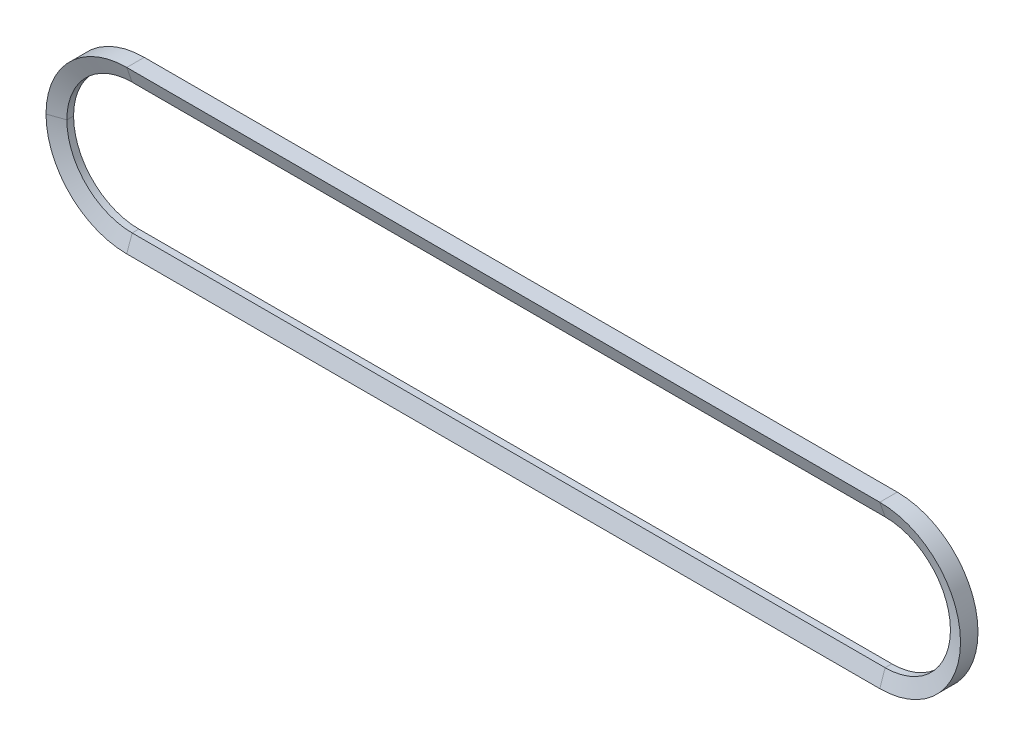
SolidWorks part; units mm, degrees
material "AISI 304"
ref_plane "Front Plane" through (0, 0, 0) normal (0, 0, 1) x (1, 0, 0)
ref_plane "Top Plane" through (0, 0, 0) normal (0, 1, 0) x (1, 0, 0)
ref_plane "Right Plane" through (0, 0, 0) normal (1, 0, 0) x (0, 0, -1)
other "Configuration Table"
sketch "Sketch1" plane through (0, 0, 0) normal (0, 0, 1) x (1, 0, 0)
  line L0 (-280, 0) -> (280, 0) construction
  line L1 (-280, 48.55) -> (280, 48.55)
  line L2 (-280, -48.55) -> (280, -48.55)
  line L3 (-280, 0) -> (-328.55, 0) construction
  arc A0 (280, -48.55) -> (280, 48.55) centre (280, 0) ccw
  arc A1 (-280, 48.55) -> (-280, -48.55) centre (-280, 0) ccw
  point P4 (0, 0)
  dimension "D2" = 97.1
  dimension "D3" = 97.1
  dimension "D1" = 560
sketch "Sketch2" plane through (0, 0, 0) normal (0, 1, 0) x (1, 0, 0)
  line L0 (-328.55, 2.5) -> (-328.55, -2.5)
  line L3 (-280, 0) -> (-328.55, 0) construction
  line L4 (-328.55, 0) -> (-340.05, 0) construction
  line L5 (-340.05, 6.5) -> (-340.05, -6.5)
  line L6 (-340.05, -6.5) -> (-328.55, -2.5)
  line L7 (-340.05, 6.5) -> (-328.55, 2.5)
  point P3 (-328.55, 0)
  point P11 (-340.05, 0)
  dimension "D1" = 5
  dimension "D2" = 0
  dimension "D3" = 13
  dimension "D4" = 11.5
sweep "Sweep1" add profiles "Sketch2" path "Sketch1"
